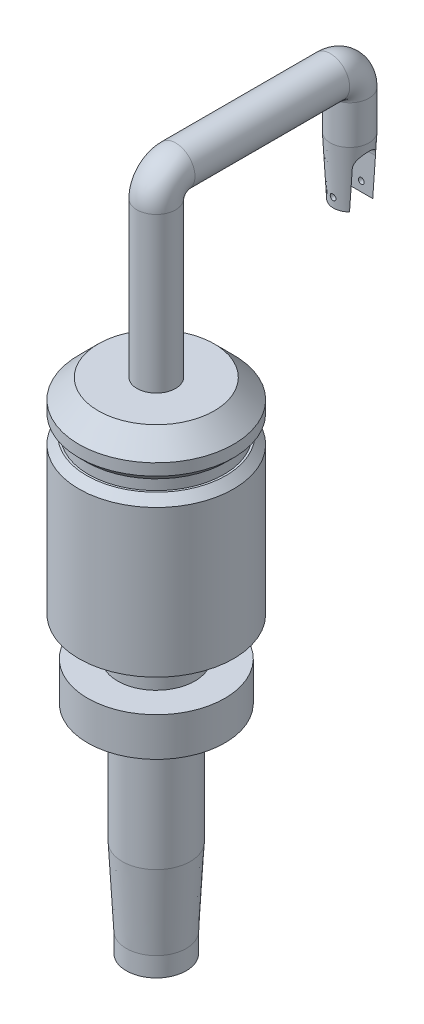
from build123d import *

# Parameters (mm, degrees)
SKETCH1_R           = 15.5
BOSS_EXTRUDE1_DEPTH = 40
BOSS_EXTRUDE1_DRAFT = -3
SKETCH2_R           = 15.5
BOSS_EXTRUDE2_DEPTH = 10
SKETCH3_R           = 17.596311171
BOSS_EXTRUDE3_DEPTH = 62
SKETCH4_R           = 35.468367634
BOSS_EXTRUDE4_DEPTH = 20
SKETCH5_R           = 20
BOSS_EXTRUDE5_DEPTH = 20
SKETCH6_R           = 40
BOSS_EXTRUDE6_DEPTH = 80
SKETCH7_R           = 35
BOSS_EXTRUDE7_DEPTH = 6
SKETCH8_R           = 40
BOSS_EXTRUDE8_DEPTH = 20
CHAMFER1_SIZE       = 10
CHAMFER2_SIZE       = 4
CHAMFER4_SIZE       = 4
SKETCH12_W          = 10
SKETCH12_H          = 80
SKETCH15_R          = 10
SKETCH17_R          = 10
BOSS_EXTRUDE9_DEPTH = 30
BOSS_EXTRUDE9_TAPER = 3
CUT_EXTRUDE1_DEPTH  = 12.5
SKETCH20_R          = 1.5
CUT_EXTRUDE2_DEPTH  = 12.5


with BuildPart() as part:
    # Sketch1 → Boss-Extrude1 (with draft: the straight prism first)
    with BuildSketch(Plane(origin=(0, 0, 0), x_dir=(1, 0, 0), z_dir=(0, 1, 0))):
        Circle(SKETCH1_R)
    extrude(amount=BOSS_EXTRUDE1_DEPTH)
    # Boss-Extrude1: the draft: its side faces are tilted about the plane it starts from
    boss_extrude1_sides = [part.faces().sort_by_distance(p)[0] for p in [
        (-15.5, 20, 0),
    ]]
    draft(boss_extrude1_sides, Plane(origin=(0, 0, 0), x_dir=(1, 0, 0), z_dir=(0, 1, 0)), BOSS_EXTRUDE1_DRAFT)

    # Sketch2 → Boss-Extrude2 (add)
    with BuildSketch(Plane.XZ):
        with Locations(Location((0, 0, 0), (0, 0, 270))):
            Circle(SKETCH2_R)
    extrude(amount=BOSS_EXTRUDE2_DEPTH)

    # Sketch3 → Boss-Extrude3 (add)
    with BuildSketch(Plane(origin=(0, 40, 0), x_dir=(1, 0, 0), z_dir=(0, 1, 0))):
        with Locations(Location((0, 0, 0), (0, 0, 270))):
            Circle(SKETCH3_R)
    extrude(amount=BOSS_EXTRUDE3_DEPTH)

    # Sketch4 → Boss-Extrude4 (add)
    with BuildSketch(Plane(origin=(0, 102, 0), x_dir=(1, 0, 0), z_dir=(0, 1, 0))):
        with Locations(Location((0, 0, 0), (0, 0, 270))):
            Circle(SKETCH4_R)
    extrude(amount=BOSS_EXTRUDE4_DEPTH)

    # Sketch5 → Boss-Extrude5 (add)
    with BuildSketch(Plane(origin=(0, 122, 0), x_dir=(1, 0, 0), z_dir=(0, 1, 0))):
        with Locations(Location((0, 0, 0), (0, 0, 270))):
            Circle(SKETCH5_R)
    extrude(amount=BOSS_EXTRUDE5_DEPTH)

    # Sketch6 → Boss-Extrude6 (add)
    with BuildSketch(Plane(origin=(0, 142, 0), x_dir=(1, 0, 0), z_dir=(0, 1, 0))):
        with Locations(Location((0, 0, 0), (0, 0, 270))):
            Circle(SKETCH6_R)
    extrude(amount=BOSS_EXTRUDE6_DEPTH)

    # Sketch7 → Boss-Extrude7 (add)
    with BuildSketch(Plane(origin=(0, 222, 0), x_dir=(1, 0, 0), z_dir=(0, 1, 0))):
        with Locations(Location((0, 0, 0), (0, 0, 270))):
            Circle(SKETCH7_R)
    extrude(amount=BOSS_EXTRUDE7_DEPTH)

    # Sketch8 → Boss-Extrude8 (add)
    with BuildSketch(Plane(origin=(0, 228, 0), x_dir=(1, 0, 0), z_dir=(0, 1, 0))):
        with Locations(Location((0, 0, 0), (0, 0, 270))):
            Circle(SKETCH8_R)
    extrude(amount=BOSS_EXTRUDE8_DEPTH)

    # Chamfer1
    chamfer1_edges = [part.edges().sort_by_distance(p)[0] for p in [
        (0, 248, -40),
    ]]
    chamfer(chamfer1_edges, length=CHAMFER1_SIZE)

    # Chamfer2
    chamfer2_edges = [part.edges().sort_by_distance(p)[0] for p in [
        (0, 222, -40),
    ]]
    chamfer(chamfer2_edges, length=CHAMFER2_SIZE)

    # Chamfer4
    chamfer4_edges = [part.edges().sort_by_distance(p)[0] for p in [
        (0, 228, -40),
    ]]
    chamfer(chamfer4_edges, length=CHAMFER4_SIZE)

    # Sketch12 → Revolve1 (revolve)
    with BuildSketch(Plane(origin=(0, 0, 0), x_dir=(0, 0, -1), z_dir=(1, 0, 0))):
        with Locations((-5, 288)):
            Rectangle(SKETCH12_W, SKETCH12_H)
    revolve(axis=Axis((0, 389.365885341, 0), (0, -1, 0)))

    # Sweep1: sweep along a path in Sketch14
    with BuildLine(Plane(origin=(0, 0, 0), x_dir=(0, 0, -1), z_dir=(1, 0, 0))) as sweep1_path:
        Line((100, 308), (100, 328))
        ThreePointArc((100, 328), (97.071067812, 335.071067812), (90, 338))
        Line((90, 338), (10, 338))
        ThreePointArc((10, 338), (2.928932188, 335.071067812), (0, 328))
    # Sketch15 → Sweep1 (sweep)
    with BuildSketch(Plane(origin=(0, 328, 0), x_dir=(1, 0, 0), z_dir=(0, 1, 0))):
        Circle(SKETCH15_R)
    sweep(path=sweep1_path.line)

    # Sketch17 → Boss-Extrude9 (add)
    with BuildSketch(Plane.XZ.offset(-308)):
        with Locations(Location((0, -100, 0), (0, 0, 270))):
            Circle(SKETCH17_R)
    extrude(amount=BOSS_EXTRUDE9_DEPTH, taper=BOSS_EXTRUDE9_TAPER)

    # Sketch19 → Cut-Extrude1 (cut, symmetric)
    with BuildSketch(Plane(origin=(0, 0, 0), x_dir=(0, 0, -1), z_dir=(1, 0, 0))):
        with BuildLine():
            Line((94, 278), (94, 298))
            ThreePointArc((94, 298), (100, 304), (106, 298))
            Line((106, 298), (106, 278))
            Line((106, 278), (94, 278))
        make_face()
    extrude(amount=CUT_EXTRUDE1_DEPTH, both=True, mode=Mode.SUBTRACT)

    # Sketch20 → Cut-Extrude2 (cut, symmetric)
    with BuildSketch(Plane.XY.offset(-99.984104739)):
        with Locations(Location((0, 283, 0), (0, 0, 90))):
            Circle(SKETCH20_R)
    extrude(amount=CUT_EXTRUDE2_DEPTH, both=True, mode=Mode.SUBTRACT)


solid = part.part
